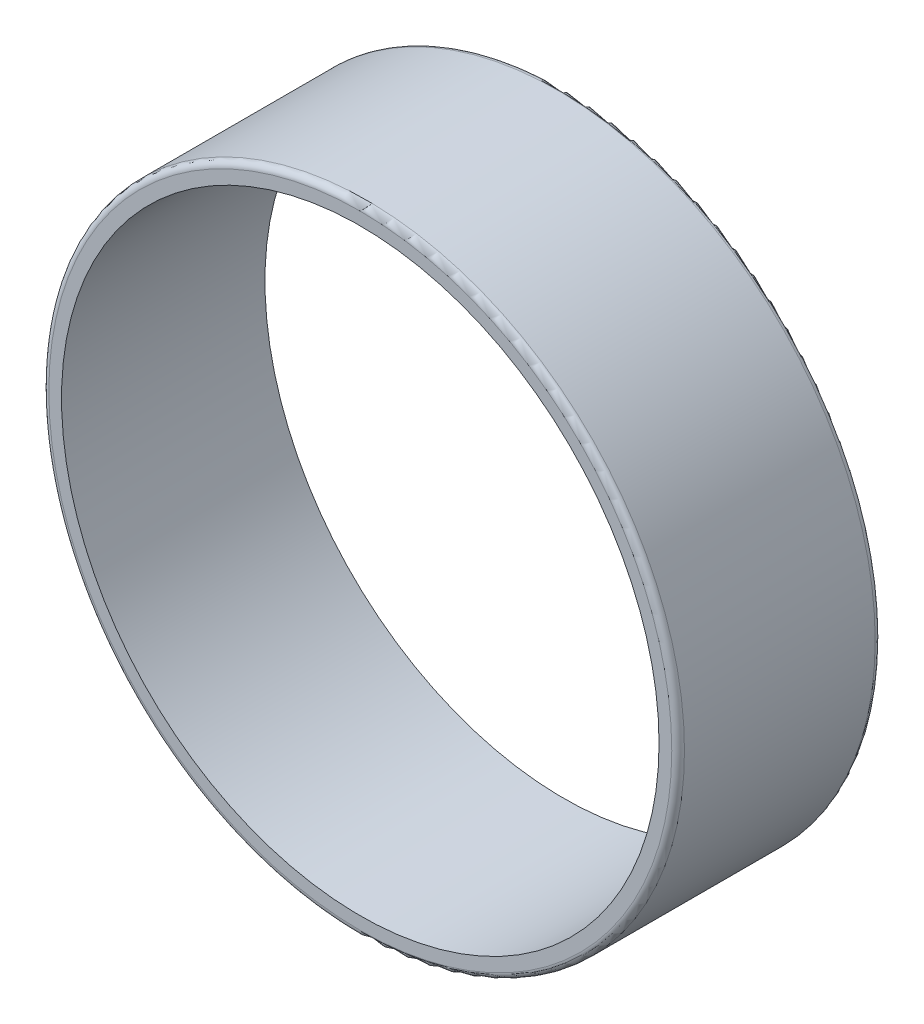
from build123d import *

# Parameters (mm, degrees)
SKETCH1_R           = 50
SKETCH1_R_2         = 47
BOSS_EXTRUDE1_DEPTH = 32
FILLET1_R           = 1


with BuildPart() as part:
    # Sketch1 → Boss-Extrude1 (new body)
    with BuildSketch(Plane.XY):
        Circle(SKETCH1_R)
        Circle(SKETCH1_R_2, mode=Mode.SUBTRACT)
    extrude(amount=BOSS_EXTRUDE1_DEPTH)

    # Fillet1
    fillet1_edges = [part.edges().sort_by_distance(p)[0] for p in [
        (-50, 0, 0),
        (-50, 0, 32),
    ]]
    fillet(fillet1_edges, radius=FILLET1_R)


solid = part.part
